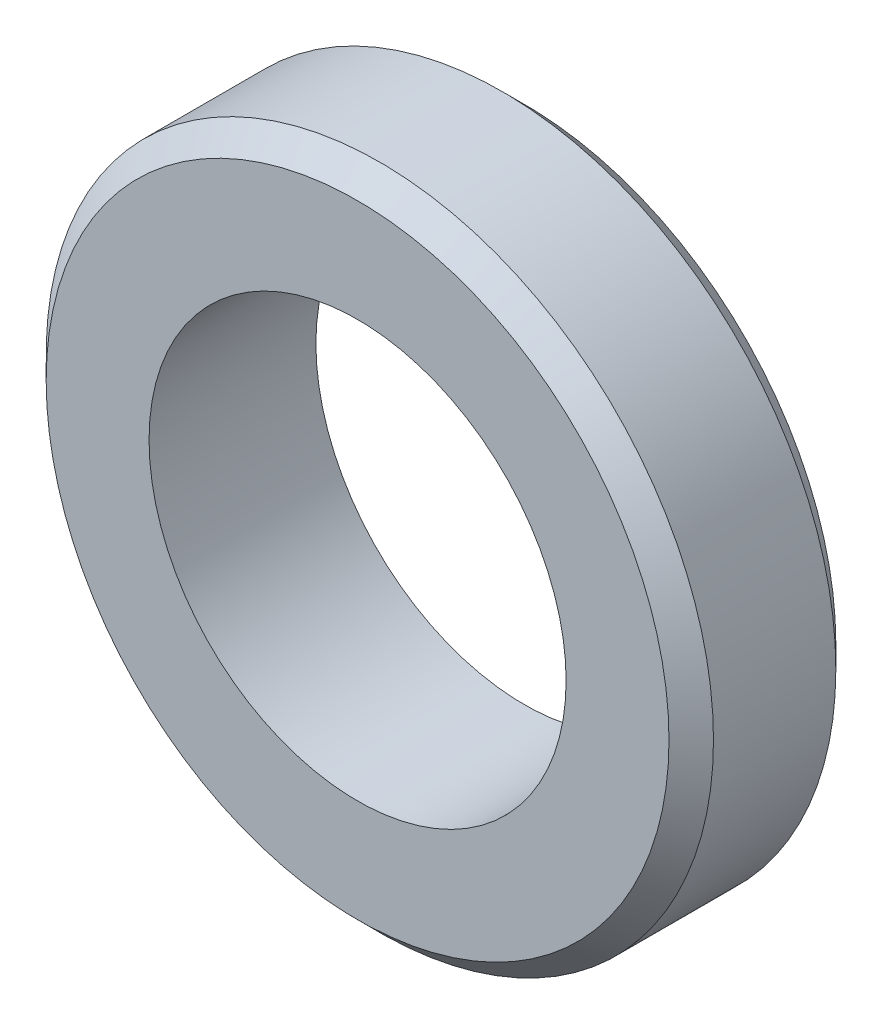
SolidWorks part; units mm, degrees
material "45"
ref_plane "Front Plane" through (0, 0, 0) normal (0, 0, 1) x (1, 0, 0)
ref_plane "Top Plane" through (0, 0, 0) normal (0, 1, 0) x (1, 0, 0)
ref_plane "Right Plane" through (0, 0, 0) normal (1, 0, 0) x (0, 0, -1)
sketch "Sketch1" plane through (0, 0, 0) normal (0, 0, 1) x (1, 0, 0)
  circle A0 centre (0, 0) radius 30
  dimension "D1" = 60
extrude "Boss-Extrude1" add sketch "Sketch1" along normal blind 15
sketch "Sketch2" plane through (0, 0, 15) normal (0, 0, 1) x (1, 0, 0)
  circle A0 centre (0, 0) radius 17.5
  dimension "D1" = 35
extrude "Cut-Extrude1" cut sketch "Sketch2" against normal blind 15
chamfer "Chamfer1" distance 2 angle 45 2 edges at (30, 0, 0) (30, 0, 15)
hole_wizard "M42 Tapped Hole4" positions "Sketch6" profile "Sketch7" tap size "M42" standard "GB"
sketch "Sketch6" plane through (0, 0, 15) normal (0, 0, 1) x (1, 0, 0)
  point P0 (0, 0)
sketch "Sketch7" plane through (0, 0, 15) normal (1, 0, 0) x (0, -1, 0)
  line L0 (0, 0) -> (0, 117.7661)
  line L1 (0, 117.7661) -> (18.75, 106.5)
  line L2 (18.75, 106.5) -> (18.75, 0)
  line L5 (18.75, 0) -> (0, 0)
  line L10 (0, 117.7661) -> (-18.75, 106.5) construction
  line L11 (0, -6.35) -> (0, 107.95) construction
  dimension "螺纹孔钻头直径" = 37.5
  dimension "螺纹孔钻头深度" = 106.5
  dimension "导头角度" = 118
cosmetic thread "Hole Thread1" parameters "D1"=15, "D2"=42
